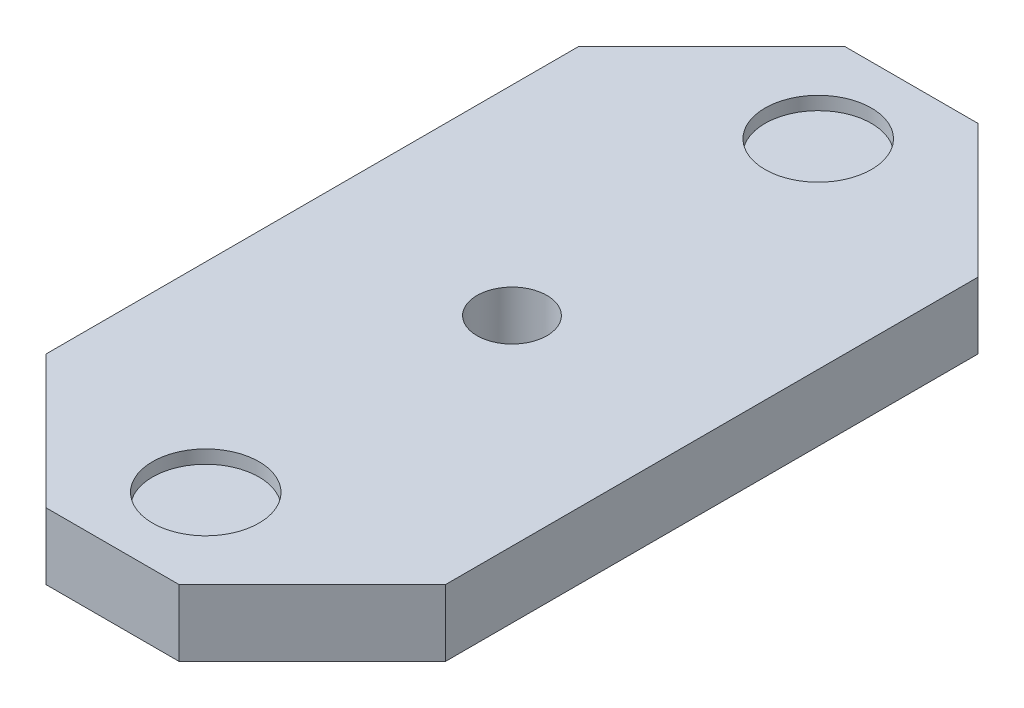
SolidWorks part; units mm, degrees
ref_plane "前视基准面" through (0, 0, 0) normal (0, 0, 1) x (1, 0, 0)
ref_plane "上视基准面" through (0, 0, 0) normal (0, 1, 0) x (1, 0, 0)
ref_plane "右视基准面" through (0, 0, 0) normal (1, 0, 0) x (0, 0, -1)
sketch "草图1" plane through (0, 0, 0) normal (0, 1, 0) x (1, 0, 0)
  line L1 (-30, -60) -> (30, -60)
  line L2 (-30, -60) -> (-30, 60)
  line L3 (-30, 60) -> (30, 60)
  line L4 (30, -60) -> (30, 60)
  line L5 (-30, -60) -> (30, 60) construction
  line L6 (-30, 60) -> (30, -60) construction
  point P0 (0, 0)
  dimension "D1" = 120
  dimension "D2" = 60
extrude "凸台-拉伸1" add sketch "草图1" along normal blind 10
sketch "草图2" plane through (0, 10, 0) normal (0, 1, 0) x (1, 0, 0)
  circle A0 centre (0, 46) radius 8
  circle A1 centre (0, -46) radius 8
extrude "切除-拉伸1" cut sketch "草图2" against normal blind 2
chamfer "倒角1" distance 20 angle 45 4 edges at (-30, 5, 60) (30, 5, 60) (30, 5, -60) (-30, 5, -60)
sketch "草图3" plane through (0, 10, 0) normal (0, 1, 0) x (1, 0, 0)
  circle A0 centre (0, 0) radius 5.25
  dimension "D1" = 10.5
extrude "切除-拉伸2" cut sketch "草图3" against normal up to next
equation "\"D3@草图2\"=\"D2@草图2\""
